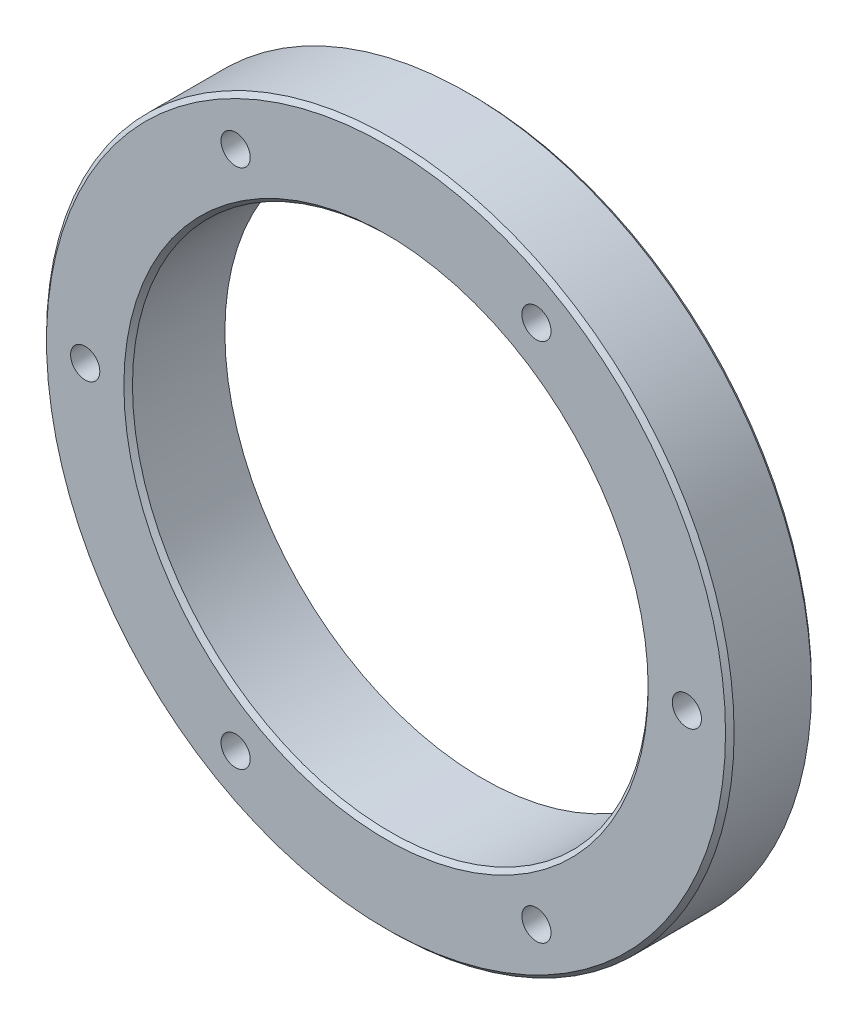
from build123d import *

# Parameters (mm, degrees)
SKETCH1_R                  = 80
SKETCH1_R_2                = 60
BOSS_EXTRUDE1_DEPTH        = 20
M8X1_25_TAPPED_HOLE2_D     = 6.8
M8X1_25_TAPPED_HOLE2_DEPTH = 18
M8X1_25_TAPPED_HOLE2_TIP   = 2.042926105
CHAMFER1_SIZE              = 1
BOSS_EXTRUDE2_START        = 2.5
SKETCH6_R                  = 75
SKETCH6_R_2                = 60
BOSS_EXTRUDE2_DEPTH        = 2.5


with BuildPart() as part:
    # Sketch1 → Boss-Extrude1 (new body)
    with BuildSketch(Plane.XY):
        Circle(SKETCH1_R)
        Circle(SKETCH1_R_2, mode=Mode.SUBTRACT)
    extrude(amount=BOSS_EXTRUDE1_DEPTH)

    # M8x1.25 Tapped Hole2
    with Locations(Plane(origin=(-35, 60.621778265, 20), x_dir=(1, 0, 0), z_dir=(0, 0, 1))):
        with Locations((0, 0), (-35, -60.621778265), (0, -121.24355653), (70, -121.24355653), (105, -60.621778265), (70, 0)):
            Hole(M8X1_25_TAPPED_HOLE2_D / 2, depth=M8X1_25_TAPPED_HOLE2_DEPTH)
            with Locations((0, 0, -(M8X1_25_TAPPED_HOLE2_DEPTH + M8X1_25_TAPPED_HOLE2_TIP / 2))):  # 118° drill point
                Cone(0, M8X1_25_TAPPED_HOLE2_D / 2, M8X1_25_TAPPED_HOLE2_TIP, mode=Mode.SUBTRACT)

    # Chamfer1
    chamfer1_edges = [part.edges().sort_by_distance(p)[0] for p in [
        (-80, 0, 0),
        (-80, 0, 20),
        (-60, 0, 20),
    ]]
    chamfer(chamfer1_edges, length=CHAMFER1_SIZE)

    # Sketch6 → Boss-Extrude2 (add)
    with BuildSketch(Plane(origin=(0, 0, 0), x_dir=(-1, 0, 0), z_dir=(0, 0, -1)).offset(BOSS_EXTRUDE2_START)):
        with Locations(Location((0, 0, 0), (0, 0, 180))):
            Circle(SKETCH6_R)
        Circle(SKETCH6_R_2, mode=Mode.SUBTRACT)
    extrude(amount=-BOSS_EXTRUDE2_DEPTH)


solid = part.part
